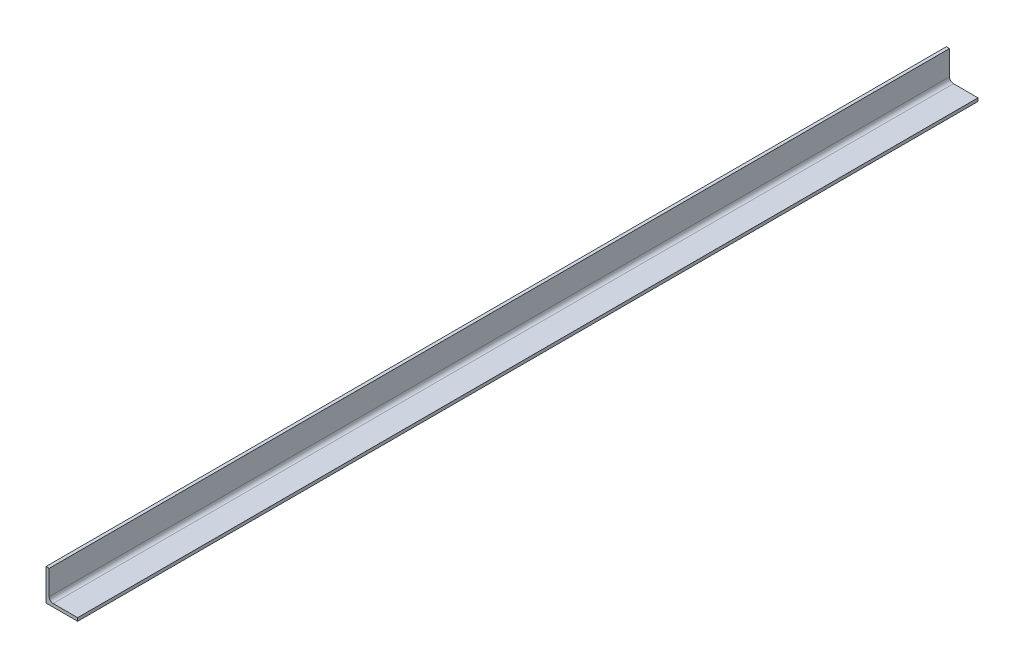
SolidWorks part; units mm, degrees
material "热轧等边角钢 Q235A"
ref_plane "前视基准面" through (0, 0, 0) normal (0, 0, 1) x (1, 0, 0)
ref_plane "上视基准面" through (0, 0, 0) normal (0, 1, 0) x (1, 0, 0)
ref_plane "右视基准面" through (0, 0, 0) normal (1, 0, 0) x (0, 0, -1)
sketch "草图1" plane through (0, 0, 0) normal (0, 0, 1) x (1, 0, 0)
  line L0 (0, 0) -> (0, 40)
  line L1 (0, 40) -> (3.99, 40)
  line L2 (4, 39.99) -> (4, 9)
  line L3 (9, 4) -> (39.99, 4)
  line L4 (40, 3.99) -> (40, 0)
  line L5 (40, 0) -> (0, 0)
  arc A0 (4, 39.99) -> (3.99, 40) centre (3.99, 39.99) ccw
  arc A1 (9, 4) -> (4, 9) centre (9, 9) cw
  arc A2 (40, 3.99) -> (39.99, 4) centre (39.99, 3.99) ccw
  point P9 (4, 40)
  point P14 (40, 4)
extrude "拉伸1" add sketch "草图1" along normal blind 1138
equation "\"D2@草图1\" = \"D1@草图1\""
equation "\"D4@草图1\" = \"D3@草图1\""
equation "\"D7@草图1\" = \"D5@草图1\""
